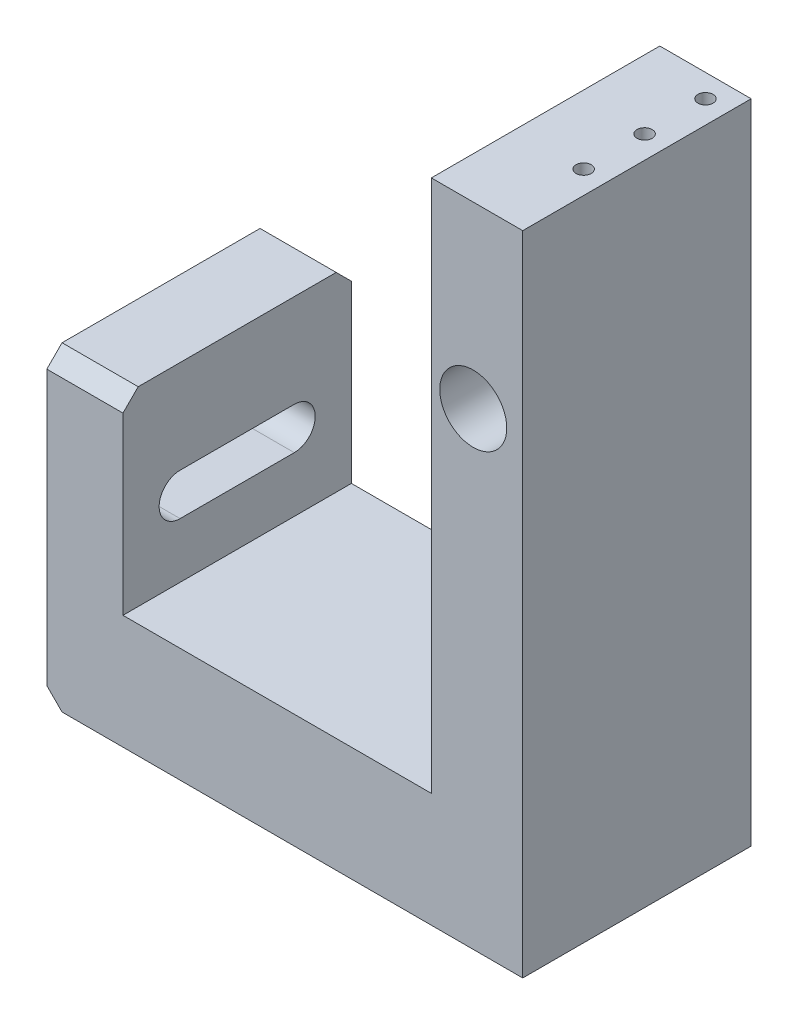
from build123d import *

# Parameters (mm, degrees)
BOSS_EXTRUDE1_DEPTH     = 30
SKETCH2_R               = 1
CUT_EXTRUDE1_DEPTH      = 25
SKETCH3_R               = 3
CUT_EXTRUDE2_DEPTH      = 28
SKETCH4_R               = 3
CUT_EXTRUDE3_DEPTH      = 61.5
CUT_EXTRUDE4_DEPTH      = 20
CHAMFER1_SIZE           = 2
G1_8_TAPPED_HOLE1_D     = 8.8
G1_8_TAPPED_HOLE1_DEPTH = 12.72
G1_8_TAPPED_HOLE1_TIP   = 2.643786724
G1_8_TAPPED_HOLE2_D     = 8.8
G1_8_TAPPED_HOLE2_DEPTH = 10.72
G1_8_TAPPED_HOLE2_TIP   = 2.643786724


with BuildPart() as part:
    # Sketch1 → Boss-Extrude1 (new body)
    with BuildSketch(Plane.XY):
        Polygon((-10, 40), (-10, 0), (52.5, 0), (52.5, 85), (40.5, 85), (40.5, 15), (0, 15), (0, 40), align=None)
    extrude(amount=BOSS_EXTRUDE1_DEPTH)

    # Sketch2 → Cut-Extrude1 (cut)
    with BuildSketch(Plane(origin=(0, 85, 0), x_dir=(1, 0, 0), z_dir=(0, 1, 0))):
        with Locations(Location((49.5, -3, 0), (0, 0, 270))):
            Circle(SKETCH2_R)
        with Locations(Location((49.5, -11, 0), (0, 0, 270))):
            Circle(SKETCH2_R)
        with Locations(Location((49.5, -19, 0), (0, 0, 270))):
            Circle(SKETCH2_R)
    extrude(amount=-CUT_EXTRUDE1_DEPTH, mode=Mode.SUBTRACT)

    # Sketch3 → Cut-Extrude2 (cut)
    with BuildSketch(Plane.XY.offset(30)):
        with Locations((46, 61.5)):
            Circle(SKETCH3_R)
    extrude(amount=-CUT_EXTRUDE2_DEPTH, mode=Mode.SUBTRACT)

    # Sketch4 → Cut-Extrude3 (cut)
    with BuildSketch(Plane.XZ):
        with Locations(Location((46, 15, 0), (0, 0, 270))):
            Circle(SKETCH4_R)
    extrude(amount=-CUT_EXTRUDE3_DEPTH, mode=Mode.SUBTRACT)

    # Sketch5 → Cut-Extrude4 (cut)
    with BuildSketch(Plane.ZY.offset(10)):
        with BuildLine():
            Line((7.5, 27.75), (22.5, 27.75))
            ThreePointArc((22.5, 27.75), (25.25, 25), (22.5, 22.25))
            Line((22.5, 22.25), (7.5, 22.25))
            ThreePointArc((7.5, 22.25), (4.75, 25), (7.5, 27.75))
        make_face()
    extrude(amount=-CUT_EXTRUDE4_DEPTH, mode=Mode.SUBTRACT)

    # Chamfer1
    chamfer1_edges = [part.edges().sort_by_distance(p)[0] for p in [
        (-5, 40, 0),
        (-10, 0, 15),
        (-5, 40, 30),
    ]]
    chamfer(chamfer1_edges, length=CHAMFER1_SIZE)

    # G1/8 Tapped Hole1
    with Locations(Plane.XZ):
        with Locations((46, 15)):
            Hole(G1_8_TAPPED_HOLE1_D / 2, depth=G1_8_TAPPED_HOLE1_DEPTH)
            with Locations((0, 0, -(G1_8_TAPPED_HOLE1_DEPTH + G1_8_TAPPED_HOLE1_TIP / 2))):  # 118° drill point
                Cone(0, G1_8_TAPPED_HOLE1_D / 2, G1_8_TAPPED_HOLE1_TIP, mode=Mode.SUBTRACT)

    # G1/8 Tapped Hole2
    with Locations(Plane.XY.offset(30)):
        with Locations((46, 61.5)):
            Hole(G1_8_TAPPED_HOLE2_D / 2, depth=G1_8_TAPPED_HOLE2_DEPTH)
            with Locations((0, 0, -(G1_8_TAPPED_HOLE2_DEPTH + G1_8_TAPPED_HOLE2_TIP / 2))):  # 118° drill point
                Cone(0, G1_8_TAPPED_HOLE2_D / 2, G1_8_TAPPED_HOLE2_TIP, mode=Mode.SUBTRACT)


solid = part.part
